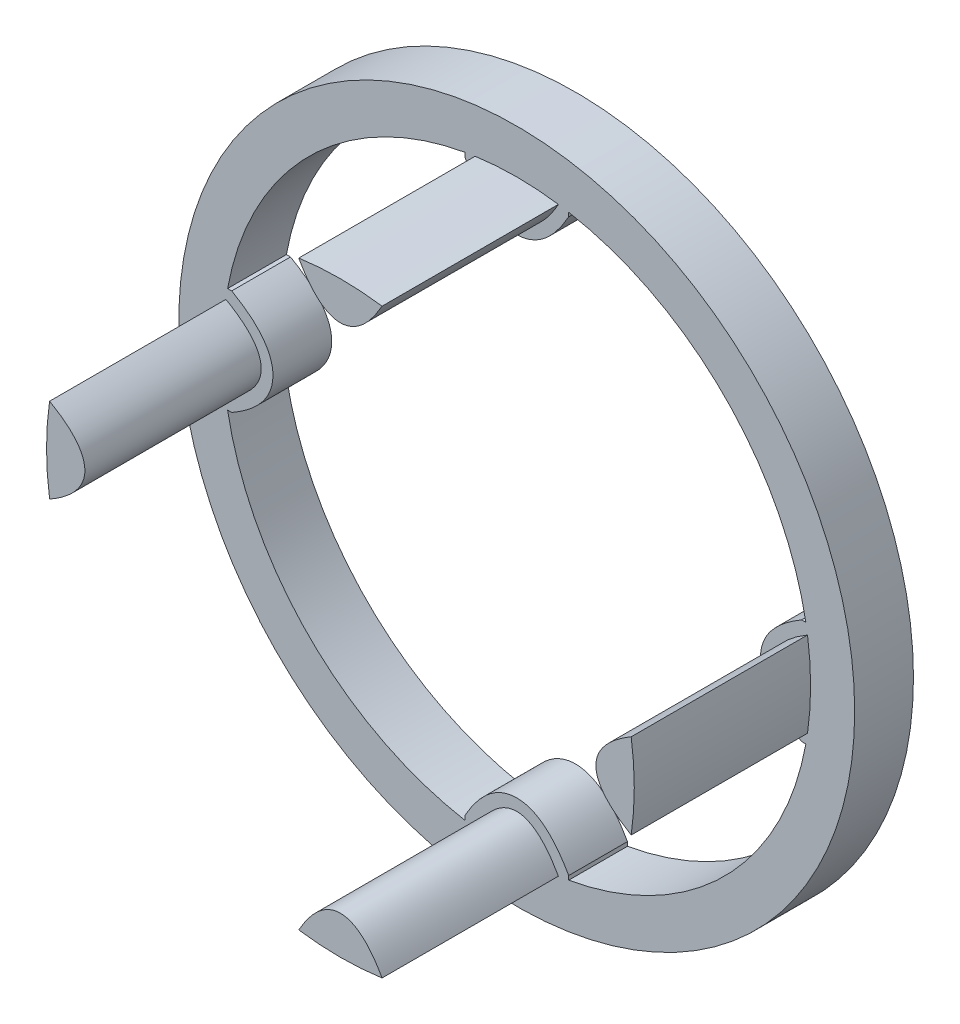
from build123d import *

# Parameters (mm, degrees)
SKETCH_1_R          = 57.5
EXTRUDE_1_DEPTH     = 40
CUT_EXTRUDE_START   = -30
SKETCH_2_R          = 60
SKETCH_2_R_2        = 50
CUT_EXTRUDE_3_DEPTH = 30
EXTRUDE_3_DEPTH     = 10
EXTRUDE_4_DEPTH     = 10
EXTRUDE_5_DEPTH     = 10
EXTRUDE_6_DEPTH     = 10


with BuildPart() as part:
    # 草图1 → 拉伸1 (new body)
    with BuildSketch(Plane.XY):
        Circle(SKETCH_1_R)
        with BuildLine():
            ThreePointArc((-7.088304974, 49.495009169), (-35.310457237, 35.400163978), (-49.476864779, 7.213865238))
            add(Edge.make_bspline(
                [(-49.476864779, -7.213865238), (-36.726647454, 0), (-49.476864779, 7.213865238)],
                knots=[5.807240593, 5.807240593, 5.807240593, 6.759130021, 6.759130021, 6.759130021], degree=2, weights=[1, 0.888860271, 1]))
            ThreePointArc((-49.476864779, -7.213865238), (-35.310457237, -35.400163978), (-7.088304974, -49.495009169))
            add(Edge.make_bspline(
                [(7.088304974, -49.495009169), (0, -36.723712512), (-7.088304974, -49.495009169)],
                knots=[5.801236265, 5.801236265, 5.801236265, 6.76513435, 6.76513435, 6.76513435], degree=2, weights=[1, 0.886093211, 1]))
            ThreePointArc((7.088304974, -49.495009169), (35.301235246, -35.409360205), (49.473100028, -7.239639051))
            add(Edge.make_bspline(
                [(49.473100028, 7.239639051), (37.120075632, 0), (49.473100028, -7.239639051)],
                knots=[2.806658856, 2.806658856, 2.806658856, 3.476526451, 3.476526451, 3.476526451], degree=2, weights=[1, 0.944432073, 1]))
            ThreePointArc((49.473100028, 7.239639051), (35.301235246, 35.409360205), (7.088304974, 49.495009169))
            add(Edge.make_bspline(
                [(-7.088304974, 49.495009169), (0, 36.723712512), (7.088304974, 49.495009169)],
                knots=[2.659643611, 2.659643611, 2.659643611, 3.623541696, 3.623541696, 3.623541696], degree=2, weights=[1, 0.886093211, 1]))
        make_face(mode=Mode.SUBTRACT)
    extrude(amount=EXTRUDE_1_DEPTH)

    # 草图2 → 拉伸3 (cut)
    with BuildSketch(Plane.XY.offset(40).offset(CUT_EXTRUDE_START)):
        Circle(SKETCH_2_R)
        Circle(SKETCH_2_R_2, mode=Mode.SUBTRACT)
    extrude(amount=CUT_EXTRUDE_3_DEPTH, mode=Mode.SUBTRACT)

    # 草图5 → 凸台-拉伸3 (add)
    with BuildSketch(Plane(origin=(0, 0, 0), x_dir=(-1, 0, 0), z_dir=(0, 0, -1))):
        with BuildLine():
            Line((49.191622289, 8.954568475), (48.492003246, 8.954568475))
            add(Edge.make_bspline(
                [(48.492003246, 8.954568475), (47.438295788, 8.358397963), (46.488698256, 7.73458393), (44.807087954, 6.419527471), (44.074256872, 5.72819176), (42.847043729, 4.252700055), (42.351776591, 3.466154718), (41.836140902, 2.208267679), (41.702698746, 1.776396531), (41.522955051, 0.896309015), (41.476864779, 0.448228181), (41.476864779, -0.448228181), (41.522955051, -0.896309015), (41.702698746, -1.776396531), (41.836140902, -2.208267679), (42.351776591, -3.466154718), (42.847043729, -4.252700055), (44.074256872, -5.72819176), (44.807087954, -6.419527471), (46.488698256, -7.73458393), (47.438295788, -8.358397963), (48.492003246, -8.954568475)],
                knots=[0, 0, 0, 0, 0.125, 0.125, 0.25, 0.25, 0.375, 0.375, 0.4375, 0.4375, 0.5, 0.5, 0.5625, 0.5625, 0.625, 0.625, 0.75, 0.75, 0.875, 0.875, 1, 1, 1, 1], degree=3))
            Line((48.492003246, -8.954568475), (49.191622289, -8.954568475))
            ThreePointArc((49.191622289, -8.954568475), (49.341920281, -8.085474816), (49.476864779, -7.213865238))
            add(Edge.make_bspline(
                [(49.476864779, 7.213865238), (36.726647454, 0), (49.476864779, -7.213865238)],
                knots=[5.807240593, 5.807240593, 5.807240593, 6.759130021, 6.759130021, 6.759130021], degree=2, weights=[1, 0.888860271, 1]))
            ThreePointArc((49.476864779, 7.213865238), (49.341920281, 8.085474816), (49.191622289, 8.954568475))
        make_face()
    extrude(amount=-EXTRUDE_3_DEPTH)

    # 草图7 → 凸台-拉伸4 (add)
    with BuildSketch(Plane(origin=(0, 0, 0), x_dir=(-1, 0, 0), z_dir=(0, 0, -1))):
        with BuildLine():
            Line((-8.837018132, -48.524441143), (-8.837018132, -49.212875455))
            ThreePointArc((-8.837018132, -49.212875455), (-7.963911028, -49.361686774), (-7.088304974, -49.495009169))
            add(Edge.make_bspline(
                [(7.088304974, -49.495009169), (0, -36.723712512), (-7.088304974, -49.495009169)],
                knots=[5.801236265, 5.801236265, 5.801236265, 6.76513435, 6.76513435, 6.76513435], degree=2, weights=[1, 0.886093211, 1]))
            ThreePointArc((7.088304974, -49.495009169), (7.963911028, -49.361686774), (8.837018132, -49.212875455))
            Line((8.837018132, -49.212875455), (8.837018132, -48.524441143))
            add(Edge.make_bspline(
                [(8.837018132, -48.524441143), (8.554002496, -48.014519989), (7.94209171, -46.989090119), (6.690805785, -45.210357531), (4.988657794, -43.371772875), (2.66472736, -41.877587359), (0, -41.303720073), (-2.66472736, -41.877587359), (-4.988657794, -43.371772875), (-6.690805785, -45.210357531), (-7.94209171, -46.989090119), (-8.554002496, -48.014519989), (-8.837018132, -48.524441143)],
                knots=[-0.481949042, -0.481949042, -0.481949042, -0.481949042, -0.421705412, -0.361461782, -0.240974521, -0.120487261, 0, 0.120487261, 0.240974521, 0.361461782, 0.421705412, 0.481949042, 0.481949042, 0.481949042, 0.481949042], degree=3))
        make_face()
    extrude(amount=-EXTRUDE_4_DEPTH)

    # 草图8 → 凸台-拉伸5 (add)
    with BuildSketch(Plane(origin=(0, 0, 0), x_dir=(-1, 0, 0), z_dir=(0, 0, -1))):
        with BuildLine():
            Line((-48.461847021, 8.965144008), (-49.189696003, 8.965144008))
            ThreePointArc((-49.189696003, 8.965144008), (-49.33894174, 8.103630542), (-49.473100028, 7.239639051))
            add(Edge.make_bspline(
                [(-49.473100028, -7.239639051), (-37.120075632, 0), (-49.473100028, 7.239639051)],
                knots=[2.806658856, 2.806658856, 2.806658856, 3.476526451, 3.476526451, 3.476526451], degree=2, weights=[1, 0.944432073, 1]))
            ThreePointArc((-49.473100028, -7.239639051), (-49.33894174, -8.103630542), (-49.189696003, -8.965144008))
            Line((-49.189696003, -8.965144008), (-48.461847021, -8.965144008))
            add(Edge.make_bspline(
                [(-48.461847021, -8.965144008), (-47.403537543, -8.344908965), (-46.455001816, -7.705959573), (-44.77995312, -6.374534454), (-44.052601357, -5.682011491), (-42.834946416, -4.212781113), (-42.343593905, -3.433612838), (-41.830983832, -2.187799789), (-41.698135209, -1.760111418), (-41.519077327, -0.888240926), (-41.473100028, -0.444200971), (-41.473100028, 0.444200971), (-41.519077327, 0.888240926), (-41.698135209, 1.760111418), (-41.830983832, 2.187799789), (-42.343593905, 3.433612838), (-42.834946416, 4.212781113), (-44.052601357, 5.682011491), (-44.77995312, 6.374534454), (-46.455001816, 7.705959573), (-47.403537543, 8.344908965), (-48.461847021, 8.965144008)],
                knots=[0, 0, 0, 0, 0.125, 0.125, 0.25, 0.25, 0.375, 0.375, 0.4375, 0.4375, 0.5, 0.5, 0.5625, 0.5625, 0.625, 0.625, 0.75, 0.75, 0.875, 0.875, 1, 1, 1, 1], degree=3))
        make_face()
    extrude(amount=-EXTRUDE_5_DEPTH)

    # 草图9 → 凸台-拉伸6 (add)
    with BuildSketch(Plane(origin=(0, 0, 0), x_dir=(-1, 0, 0), z_dir=(0, 0, -1))):
        with BuildLine():
            Line((-8.837018132, 48.524441143), (-8.837018132, 49.212875455))
            ThreePointArc((-8.837018132, 49.212875455), (-7.963911028, 49.361686774), (-7.088304974, 49.495009169))
            add(Edge.make_bspline(
                [(-7.088304974, 49.495009169), (0, 36.723712512), (7.088304974, 49.495009169)],
                knots=[5.801236265, 5.801236265, 5.801236265, 6.76513435, 6.76513435, 6.76513435], degree=2, weights=[1, 0.886093211, 1]))
            ThreePointArc((7.088304974, 49.495009169), (7.963911028, 49.361686774), (8.837018132, 49.212875455))
            Line((8.837018132, 49.212875455), (8.837018132, 48.524441143))
            add(Edge.make_bspline(
                [(-8.837018132, 48.524441143), (-8.25251339, 47.471314411), (-7.640371758, 46.521874102), (-6.348477364, 44.839518065), (-5.668669979, 44.105757745), (-4.214861328, 42.875160029), (-3.438384565, 42.377297638), (-2.192699526, 41.857811777), (-1.764410814, 41.7231382), (-0.890706349, 41.541621262), (-0.445433319, 41.495009169), (0.445433319, 41.495009169), (0.890706349, 41.541621262), (1.764410814, 41.7231382), (2.192699526, 41.857811777), (3.438384565, 42.377297638), (4.214861328, 42.875160029), (5.668669979, 44.105757745), (6.348477364, 44.839518065), (7.640371758, 46.521874102), (8.25251339, 47.471314411), (8.837018132, 48.524441143)],
                knots=[0, 0, 0, 0, 0.125, 0.125, 0.25, 0.25, 0.375, 0.375, 0.4375, 0.4375, 0.5, 0.5, 0.5625, 0.5625, 0.625, 0.625, 0.75, 0.75, 0.875, 0.875, 1, 1, 1, 1], degree=3))
        make_face()
    extrude(amount=-EXTRUDE_6_DEPTH)


solid = part.part
